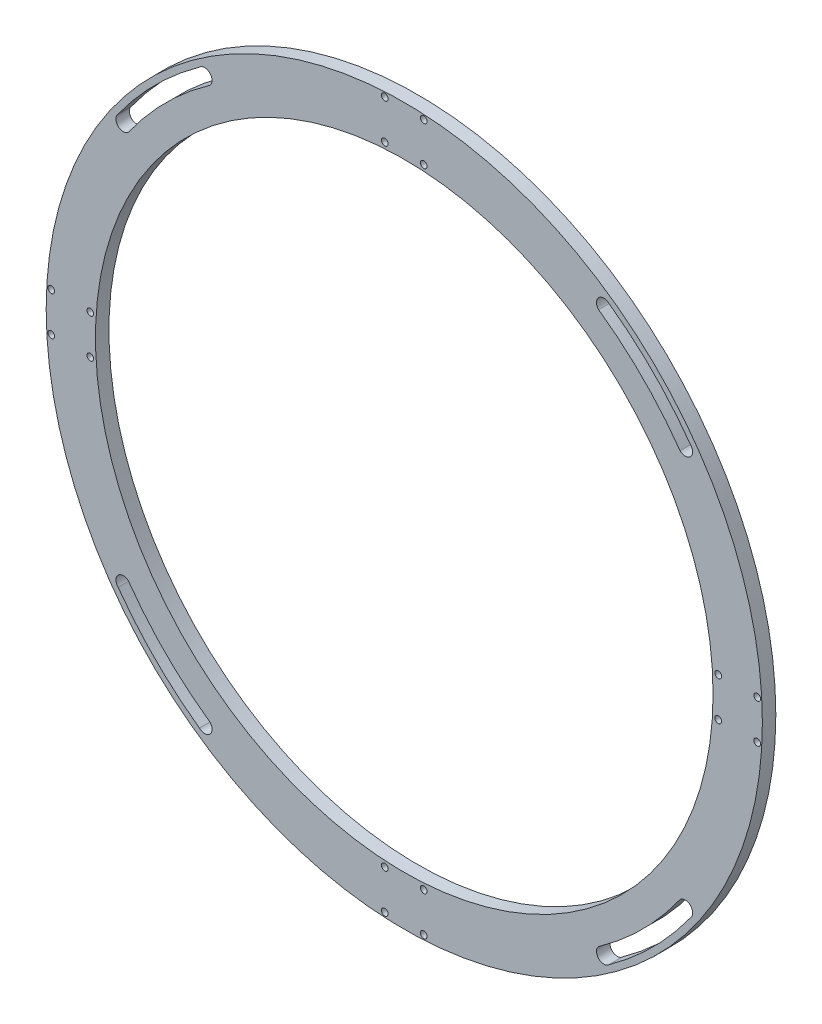
SolidWorks part; units mm, degrees
ref_plane "Front Plane" through (0, 0, 0) normal (0, 0, 1) x (1, 0, 0)
ref_plane "Top Plane" through (0, 0, 0) normal (0, 1, 0) x (1, 0, 0)
ref_plane "Right Plane" through (0, 0, 0) normal (1, 0, 0) x (0, 0, -1)
sketch "Sketch1" plane through (0, 0, 0) normal (0, 0, 1) x (1, 0, 0)
  circle A0 centre (0, 0) radius 137.7461
  circle A1 centre (0, 0) radius 159.7461
  circle A2 centre (8.7, -157.4461) radius 1.5 construction
  circle A3 centre (8.7, -140.0461) radius 1.5 construction
  circle A4 centre (-8.7, -140.0461) radius 1.5 construction
  circle A5 centre (-8.7, -157.4461) radius 1.5 construction
  circle A6 centre (157.4461, -8.7) radius 1.5 construction
  circle A7 centre (157.4461, 8.7) radius 1.5 construction
  circle A8 centre (140.0461, -8.7) radius 1.5 construction
  circle A9 centre (140.0461, 8.7) radius 1.5 construction
  circle A10 centre (8.7, 157.4461) radius 1.5 construction
  circle A11 centre (8.7, 140.0461) radius 1.5 construction
  circle A12 centre (-8.7, 140.0461) radius 1.5 construction
  circle A13 centre (-8.7, 157.4461) radius 1.5 construction
  circle A14 centre (-157.4461, -8.7) radius 1.5 construction
  circle A15 centre (-140.0461, -8.7) radius 1.5 construction
  circle A16 centre (-140.0461, 8.7) radius 1.5 construction
  circle A17 centre (-157.4461, 8.7) radius 1.5 construction
  circle A18 centre (8.7, -157.4461) radius 1.5
  circle A19 centre (8.7, -140.0461) radius 1.5
  circle A20 centre (-8.7, -140.0461) radius 1.5
  circle A21 centre (-8.7, -157.4461) radius 1.5
  circle A22 centre (157.4461, -8.7) radius 1.5
  circle A23 centre (157.4461, 8.7) radius 1.5
  circle A24 centre (140.0461, -8.7) radius 1.5
  circle A25 centre (140.0461, 8.7) radius 1.5
  circle A26 centre (8.7, 157.4461) radius 1.5
  circle A27 centre (8.7, 140.0461) radius 1.5
  circle A28 centre (-8.7, 140.0461) radius 1.5
  circle A29 centre (-8.7, 157.4461) radius 1.5
  circle A30 centre (-157.4461, -8.7) radius 1.5
  circle A31 centre (-140.0461, -8.7) radius 1.5
  circle A32 centre (-140.0461, 8.7) radius 1.5
  circle A33 centre (-157.4461, 8.7) radius 1.5
  arc A34 (127.6636, 91.3839) -> (91.3839, 127.6636) centre (0, 0) ccw
  arc A35 (123.0189, 86.6983) -> (86.6983, 123.0189) centre (0, 0) ccw
  arc A36 (91.3839, 127.6636) -> (86.6983, 123.0189) centre (89.0411, 125.3412) ccw
  circle A37 centre (0, 0) radius 150.5 construction
  circle A38 centre (0, 0) radius 157 construction
  arc A39 (123.0189, 86.6983) -> (127.6636, 91.3839) centre (125.3412, 89.0411) ccw
  arc A40 (91.3839, -127.6636) -> (127.6636, -91.3839) centre (0, 0) ccw
  arc A41 (86.6983, -123.0189) -> (123.0189, -86.6983) centre (0, 0) ccw
  arc A42 (127.6636, -91.3839) -> (123.0189, -86.6983) centre (125.3412, -89.0411) ccw
  arc A43 (86.6983, -123.0189) -> (91.3839, -127.6636) centre (89.0411, -125.3412) ccw
  arc A44 (-127.6636, -91.3839) -> (-91.3839, -127.6636) centre (0, 0) ccw
  arc A45 (-123.0189, -86.6983) -> (-86.6983, -123.0189) centre (0, 0) ccw
  arc A46 (-91.3839, -127.6636) -> (-86.6983, -123.0189) centre (-89.0411, -125.3412) ccw
  arc A47 (-123.0189, -86.6983) -> (-127.6636, -91.3839) centre (-125.3412, -89.0411) ccw
  arc A48 (-91.3839, 127.6636) -> (-127.6636, 91.3839) centre (0, 0) ccw
  arc A49 (-86.6983, 123.0189) -> (-123.0189, 86.6983) centre (0, 0) ccw
  arc A50 (-127.6636, 91.3839) -> (-123.0189, 86.6983) centre (-125.3412, 89.0411) ccw
  arc A51 (-86.6983, 123.0189) -> (-91.3839, 127.6636) centre (-89.0411, 125.3412) ccw
  point P54 (146.3146, 44.7329)
  point P55 (-17.6777, 17.6777)
  point P56 (140.2931, 140.2931)
  point P57 (122.6155, 157.9708)
  point P58 (17.6777, -17.6777)
  point P59 (157.9708, 122.6155)
  point P66 (146.5, 0)
  point P89 (0, 0)
  dimension "D1" = 6.5
  dimension "D2" = 4
extrude "Boss-Extrude1" add sketch "Sketch1" along normal blind 6 contours A1
